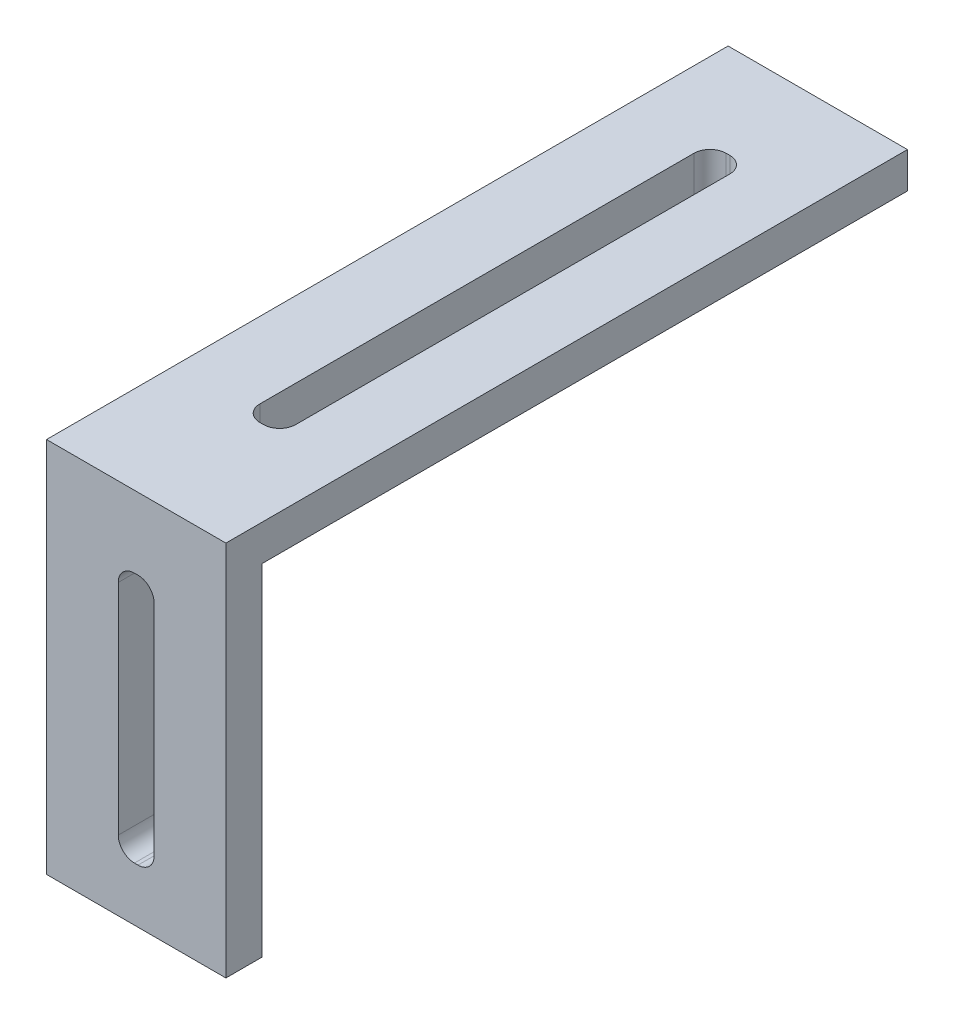
from build123d import *

# Parameters (mm, degrees)
SKETCH1_W                = 50
SKETCH1_H                = 100
BOSS_EXTRUDE1_DEPTH      = 10
CUT_EXTRUDE1_DEPTH       = 10
BOSS_EXTRUDE2_DEPTH      = 180
BOSS_EXTRUDE2_DEPTH_BACK = 10
SKETCH3_W                = 50
SKETCH3_H                = 10
CUT_EXTRUDE2_DEPTH       = 180


with BuildPart() as part:
    # Sketch1 → Boss-Extrude1 (new body)
    with BuildSketch(Plane.XY):
        Rectangle(SKETCH1_W, SKETCH1_H)
    extrude(amount=BOSS_EXTRUDE1_DEPTH)

    # Sketch2 → Cut-Extrude1 (cut)
    with BuildSketch(Plane.XY.offset(10)):
        with BuildLine():
            Line((0.5, -35), (-0.5, -35))
            ThreePointArc((-0.5, -35), (-3.681980515, -33.681980515), (-5, -30.5))
            Line((-5, -30.5), (-5, 30.5))
            ThreePointArc((-5, 30.5), (-3.681980515, 33.681980515), (-0.5, 35))
            Line((-0.5, 35), (0.5, 35))
            ThreePointArc((0.5, 35), (3.681980515, 33.681980515), (5, 30.5))
            Line((5, 30.5), (5, -30.5))
            ThreePointArc((5, -30.5), (3.681980515, -33.681980515), (0.5, -35))
        make_face()
    extrude(amount=-CUT_EXTRUDE1_DEPTH, mode=Mode.SUBTRACT)

    # Sketch3 → Boss-Extrude2 (add, two sides: drawn at the far end of the back side and taken through both)
    with BuildSketch(Plane(origin=(0, 0, 0), x_dir=(-1, 0, 0), z_dir=(0, 0, -1)).offset(-BOSS_EXTRUDE2_DEPTH_BACK)):
        with Locations((0, 50)):
            Rectangle(SKETCH3_W, SKETCH3_H)
    extrude(amount=BOSS_EXTRUDE2_DEPTH + BOSS_EXTRUDE2_DEPTH_BACK)

    # Sketch4 → Cut-Extrude2 (cut)
    with BuildSketch(Plane.XZ.offset(-45)):
        with BuildLine():
            Line((1.63487738, -153.842941115), (0.63487738, -153.842941115))
            ThreePointArc((0.63487738, -153.842941115), (-2.547103135, -152.52492163), (-3.86512262, -149.342941115))
            Line((-3.86512262, -149.342941115), (-3.86512262, -28.342941115))
            ThreePointArc((-3.86512262, -28.342941115), (-2.547103135, -25.160960599), (0.63487738, -23.842941115))
            Line((0.63487738, -23.842941115), (1.63487738, -23.842941115))
            ThreePointArc((1.63487738, -23.842941115), (4.816857896, -25.160960599), (6.13487738, -28.342941115))
            Line((6.13487738, -28.342941115), (6.13487738, -149.342941115))
            ThreePointArc((6.13487738, -149.342941115), (4.816857896, -152.52492163), (1.63487738, -153.842941115))
        make_face()
    extrude(amount=-CUT_EXTRUDE2_DEPTH, mode=Mode.SUBTRACT)


solid = part.part
